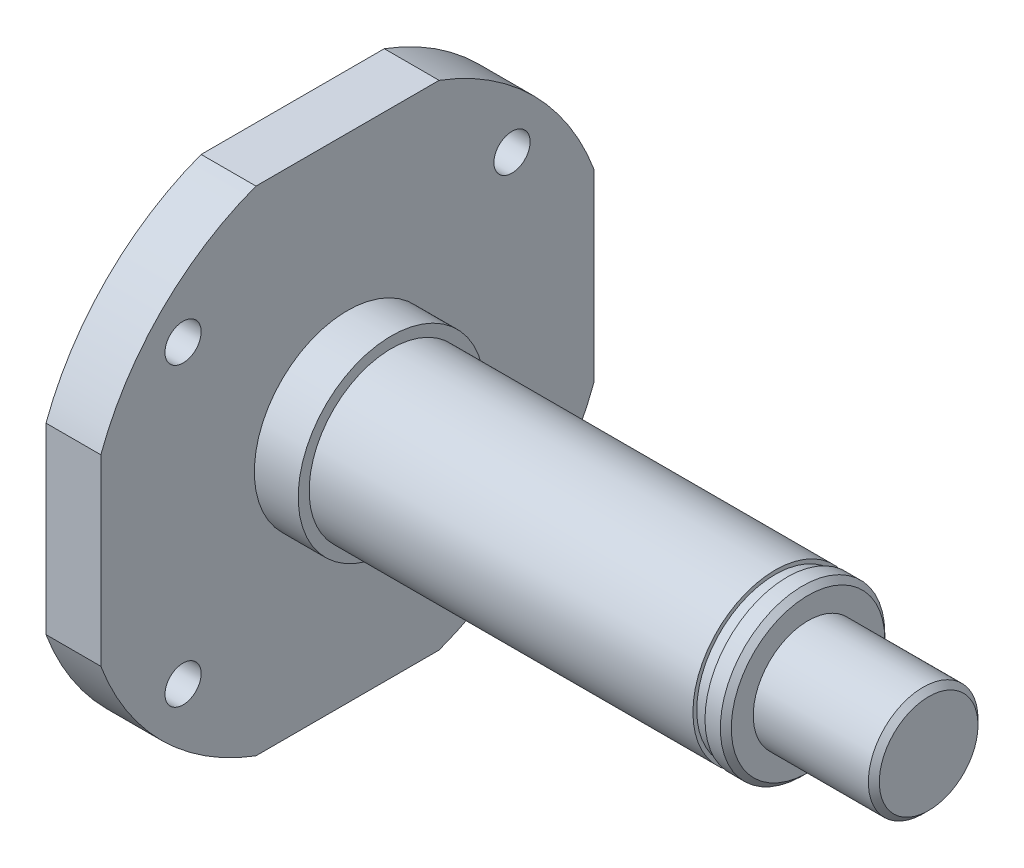
from build123d import *

# Parameters (mm, degrees)
HOLE_WIZARD_M4_1_D   = 3.3
SKETCH_4_OUTSIDE_W   = 67.858
SKETCH_4_OUTSIDE_H   = 67.858
SKETCH_4_OUTSIDE_W_2 = 45
SKETCH_4_OUTSIDE_H_2 = 45
CUT_EXTRUDE_1_DEPTH  = 10
CHAMFER_1_SIZE       = 0.5
SKETCH_5_W           = 1.1
SKETCH_5_H           = 0.35


with BuildPart() as part:
    # 草图1 → 旋转1 (revolve)
    with BuildSketch(Plane(origin=(0, 0, 0), x_dir=(1, 0, 0), z_dir=(0, 1, 0))):
        Polygon((0, 0), (0, 24), (5, 24), (5, 8.5), (9, 8.5), (9, 7.5), (47, 7.5), (47, 5), (58, 5), (58, 0), align=None)
    revolve(axis=Axis((58, 0, 0), (-1, 0, 0)))

    # M4 螺纹孔1 (through all)
    with Locations(Plane(origin=(0, 13.5, -15), x_dir=(0, 0, -1), z_dir=(-1, 0, 0))):
        with Locations((0, 0), (-30, 0), (0, 27), (-30, 27)):
            Hole(HOLE_WIZARD_M4_1_D / 2)

    # 草图4 outside → 切除-拉伸1 (cut)
    with BuildSketch(Plane.ZY):
        Rectangle(SKETCH_4_OUTSIDE_W, SKETCH_4_OUTSIDE_H)
        Rectangle(SKETCH_4_OUTSIDE_W_2, SKETCH_4_OUTSIDE_H_2, mode=Mode.SUBTRACT)
    extrude(amount=-CUT_EXTRUDE_1_DEPTH, mode=Mode.SUBTRACT)

    # 倒角1
    chamfer_1_edges = [part.edges().sort_by_distance(p)[0] for p in [
        (58, 0, 5),
        (47, 0, 7.5),
    ]]
    chamfer(chamfer_1_edges, length=CHAMFER_1_SIZE)

    # 草图5 → 切除-旋转1 (revolve, cut)
    with BuildSketch(Plane(origin=(0, 0, 0), x_dir=(1, 0, 0), z_dir=(0, 1, 0))):
        with Locations((44.55, 7.325)):
            Rectangle(SKETCH_5_W, SKETCH_5_H)
    revolve(axis=Axis((0, 0, 0), (1, 0, 0)), mode=Mode.SUBTRACT)


solid = part.part
